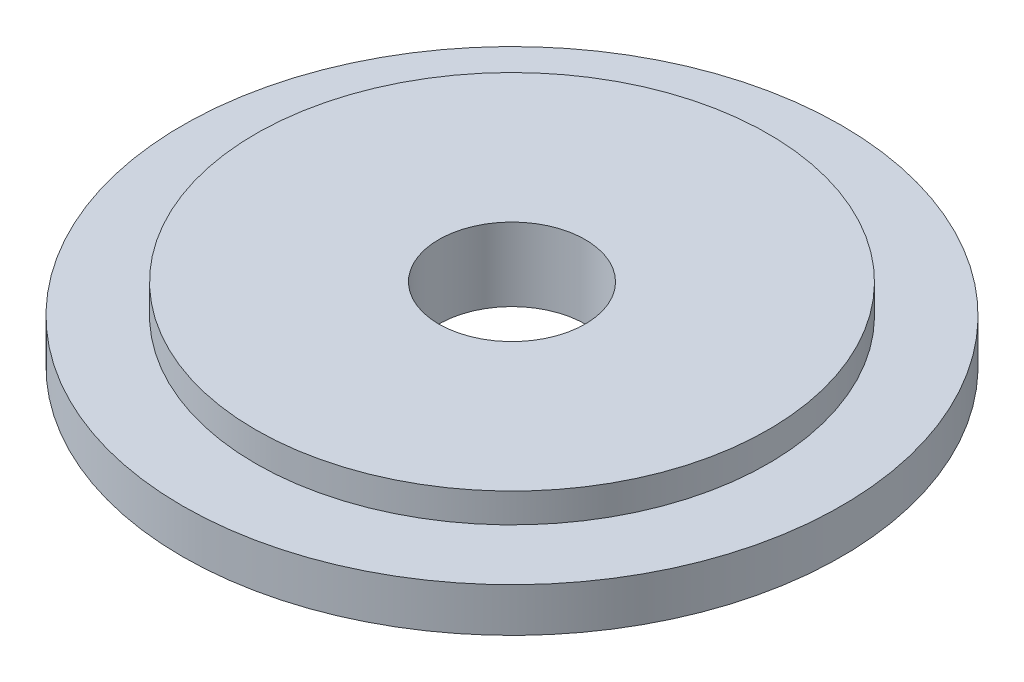
SolidWorks part; units mm, degrees
ref_plane "前视基准面" through (0, 0, 0) normal (0, 0, 1) x (1, 0, 0)
ref_plane "上视基准面" through (0, 0, 0) normal (0, 1, 0) x (1, 0, 0)
ref_plane "右视基准面" through (0, 0, 0) normal (1, 0, 0) x (0, 0, -1)
sketch "草图1" plane through (0, 0, 0) normal (0, 1, 0) x (1, 0, 0)
  circle A0 centre (0, 0) radius 22.5
extrude "凸台-拉伸1" add sketch "草图1" along normal blind 3
sketch "草图2" plane through (0, 3, 0) normal (0, 1, 0) x (1, 0, 0)
  circle A0 centre (0, 0) radius 17.5
extrude "凸台-拉伸2" add sketch "草图2" along normal blind 2
sketch "草图3" plane through (0, 5, 0) normal (0, 1, 0) x (1, 0, 0)
  circle A0 centre (0, 0) radius 5
extrude "切除-拉伸1" cut sketch "草图3" against normal through all
